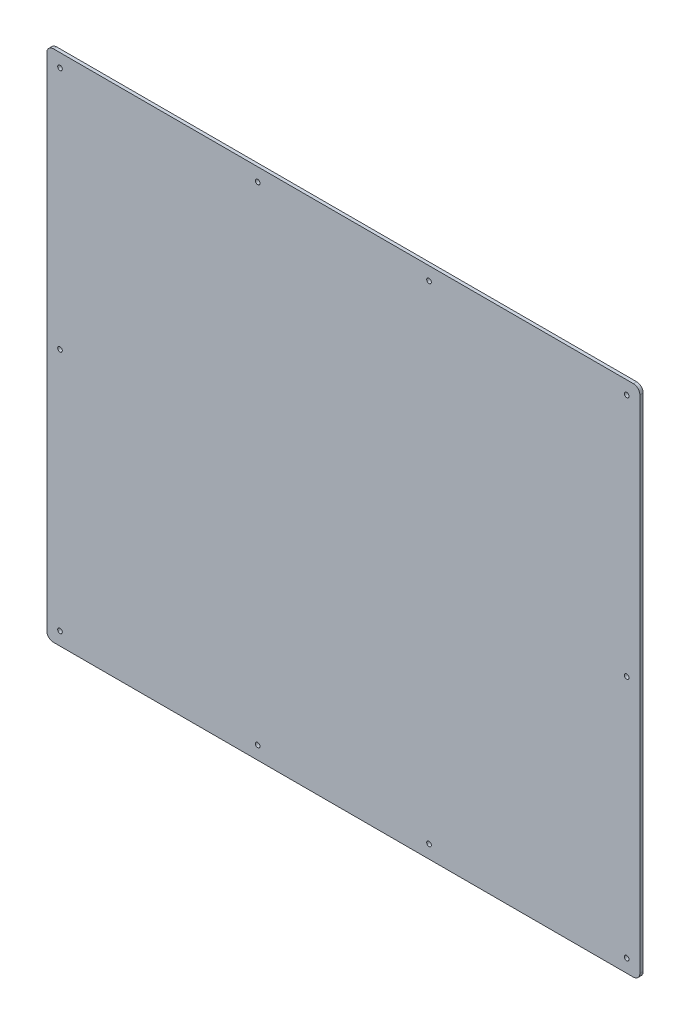
from build123d import *

# Parameters (mm, degrees)
SKETCH_1_W                = 900
SKETCH_1_H                = 780
EXTRUDE_1_DEPTH           = 5
HOLE_WIZARD_7_0_7_1_D     = 7
HOLE_WIZARD_7_0_7_1_DEPTH = 27.75
HOLE_WIZARD_7_0_7_1_TIP   = 2.103012167
FILLET_1_R                = 10


with BuildPart() as part:
    # 草图1 → 凸台-拉伸1 (new body)
    with BuildSketch(Plane.XY):
        Rectangle(SKETCH_1_W, SKETCH_1_H)
    extrude(amount=EXTRUDE_1_DEPTH)

    # Ø7.0 (7) 直径孔1
    with Locations(Plane.XY.offset(5)):
        with Locations((-430, 370), (430, 370), (430, -370), (-430, -370), (-430, 0), (430, 0), (-130, 370), (130, 370), (-130, -370), (130, -370)):
            Hole(HOLE_WIZARD_7_0_7_1_D / 2, depth=HOLE_WIZARD_7_0_7_1_DEPTH)
            with Locations((0, 0, -(HOLE_WIZARD_7_0_7_1_DEPTH + HOLE_WIZARD_7_0_7_1_TIP / 2))):  # 118° drill point
                Cone(0, HOLE_WIZARD_7_0_7_1_D / 2, HOLE_WIZARD_7_0_7_1_TIP, mode=Mode.SUBTRACT)

    # 圆角1
    fillet_1_edges = [part.edges().sort_by_distance(p)[0] for p in [
        (450, -390, 2.5),
        (-450, -390, 2.5),
        (-450, 390, 2.5),
        (450, 390, 2.5),
    ]]
    fillet(fillet_1_edges, radius=FILLET_1_R)


solid = part.part
